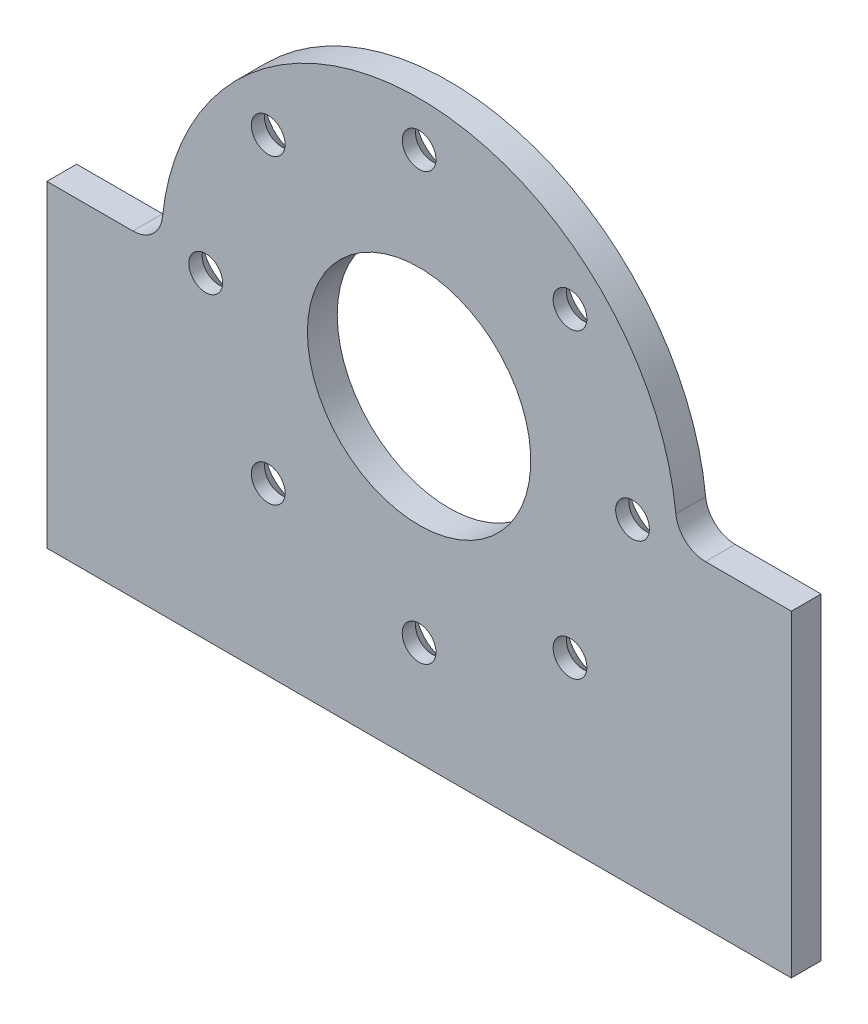
from build123d import *

# Parameters (mm, degrees)
SKETCH_1_W                  = 75
SKETCH_1_H                  = 32
EXTRUDE_1_DEPTH             = 3
SKETCH_2_R                  = 26
EXTRUDE_3_DEPTH             = 3
FILLET_1_R                  = 3
SKETCH_3_R                  = 11.25
CUT_EXTRUDE_1_DEPTH         = 57.384838388
HOLE_WIZARD_M3_1_AT_2_COUNT = 2
HOLE_WIZARD_M3_1_AT_2_PITCH = 16.455387592
HOLE_WIZARD_M3_1_AT_3_COUNT = 2
HOLE_WIZARD_M3_1_AT_3_PITCH = 30.405591591
HOLE_WIZARD_M3_1_AT_4_COUNT = 2
HOLE_WIZARD_M3_1_AT_4_PITCH = 39.726819898
HOLE_WIZARD_M3_1_AT_5_COUNT = 2
HOLE_WIZARD_M3_1_AT_5_PITCH = 43
HOLE_WIZARD_M3_1_AT_6_COUNT = 2
HOLE_WIZARD_M3_1_AT_6_PITCH = 39.726819898
HOLE_WIZARD_M3_1_AT_7_COUNT = 2
HOLE_WIZARD_M3_1_AT_7_PITCH = 30.405591591
HOLE_WIZARD_M3_1_AT_8_COUNT = 2
HOLE_WIZARD_M3_1_AT_8_PITCH = 16.455387592


with BuildPart() as part:
    # 草图1 → 凸台-拉伸1 (new body)
    with BuildSketch(Plane.XY):
        Rectangle(SKETCH_1_W, SKETCH_1_H)
    extrude(amount=EXTRUDE_1_DEPTH)

    # 草图2 → 凸台-拉伸3 (add, through all)
    with BuildSketch(Plane.XY.offset(3)):
        with Locations((0, 16)):
            Circle(SKETCH_2_R)
    extrude(amount=-EXTRUDE_3_DEPTH)

    # 圆角1
    fillet_1_edges = [part.edges().sort_by_distance(p)[0] for p in [
        (26, 16, 1.5),
        (-26, 16, 1.5),
    ]]
    fillet(fillet_1_edges, radius=FILLET_1_R)

    # 草图3 → 切除-拉伸1 (cut, through all)
    with BuildSketch(Plane(origin=(0, 0, 0), x_dir=(-1, 0, 0), z_dir=(0, 0, -1))):
        with Locations((0, 16)):
            Circle(SKETCH_3_R)
    extrude(amount=-CUT_EXTRUDE_1_DEPTH, mode=Mode.SUBTRACT)

    # 草图5 → M3 六角凹锥坑螺钉的锥形沉头孔1 (revolve, cut)
    with BuildSketch(Plane(origin=(0, 37.5, 0), x_dir=(0, 1, 0), z_dir=(1, 0, 0))):
        Polygon((0, 0), (0, 3), (1.7, 3), (1.7, 1.66), (3.36, 0), align=None)
    hole_wizard_m3_1 = revolve(axis=Axis((0, 37.5, -6.35), (0, 0, 1)), mode=Mode.SUBTRACT)

    # M3 六角凹锥坑螺钉的锥形沉头孔1 at 2: M3 六角凹锥坑螺钉的锥形沉头孔1 ×2
    with Locations(*[Vector(-0.9238795325112867, -0.38268343236508967, 0) * (i * HOLE_WIZARD_M3_1_AT_2_PITCH) for i in range(1, HOLE_WIZARD_M3_1_AT_2_COUNT)]):
        add(hole_wizard_m3_1, mode=Mode.SUBTRACT)

    # M3 六角凹锥坑螺钉的锥形沉头孔1 at 3: M3 六角凹锥坑螺钉的锥形沉头孔1 ×2
    with Locations(*[Vector(-0.7071067811865476, -0.7071067811865475, 0) * (i * HOLE_WIZARD_M3_1_AT_3_PITCH) for i in range(1, HOLE_WIZARD_M3_1_AT_3_COUNT)]):
        add(hole_wizard_m3_1, mode=Mode.SUBTRACT)

    # M3 六角凹锥坑螺钉的锥形沉头孔1 at 4: M3 六角凹锥坑螺钉的锥形沉头孔1 ×2
    with Locations(*[Vector(-0.38268343236508995, -0.9238795325112867, 0) * (i * HOLE_WIZARD_M3_1_AT_4_PITCH) for i in range(1, HOLE_WIZARD_M3_1_AT_4_COUNT)]):
        add(hole_wizard_m3_1, mode=Mode.SUBTRACT)

    # M3 六角凹锥坑螺钉的锥形沉头孔1 at 5: M3 六角凹锥坑螺钉的锥形沉头孔1 ×2
    with Locations(*[(0, -i * HOLE_WIZARD_M3_1_AT_5_PITCH, 0) for i in range(1, HOLE_WIZARD_M3_1_AT_5_COUNT)]):
        add(hole_wizard_m3_1, mode=Mode.SUBTRACT)

    # M3 六角凹锥坑螺钉的锥形沉头孔1 at 6: M3 六角凹锥坑螺钉的锥形沉头孔1 ×2
    with Locations(*[Vector(0.38268343236508967, -0.9238795325112868, 0) * (i * HOLE_WIZARD_M3_1_AT_6_PITCH) for i in range(1, HOLE_WIZARD_M3_1_AT_6_COUNT)]):
        add(hole_wizard_m3_1, mode=Mode.SUBTRACT)

    # M3 六角凹锥坑螺钉的锥形沉头孔1 at 7: M3 六角凹锥坑螺钉的锥形沉头孔1 ×2
    with Locations(*[Vector(0.7071067811865474, -0.7071067811865477, 0) * (i * HOLE_WIZARD_M3_1_AT_7_PITCH) for i in range(1, HOLE_WIZARD_M3_1_AT_7_COUNT)]):
        add(hole_wizard_m3_1, mode=Mode.SUBTRACT)

    # M3 六角凹锥坑螺钉的锥形沉头孔1 at 8: M3 六角凹锥坑螺钉的锥形沉头孔1 ×2
    with Locations(*[Vector(0.9238795325112868, -0.3826834323650898, 0) * (i * HOLE_WIZARD_M3_1_AT_8_PITCH) for i in range(1, HOLE_WIZARD_M3_1_AT_8_COUNT)]):
        add(hole_wizard_m3_1, mode=Mode.SUBTRACT)


solid = part.part
